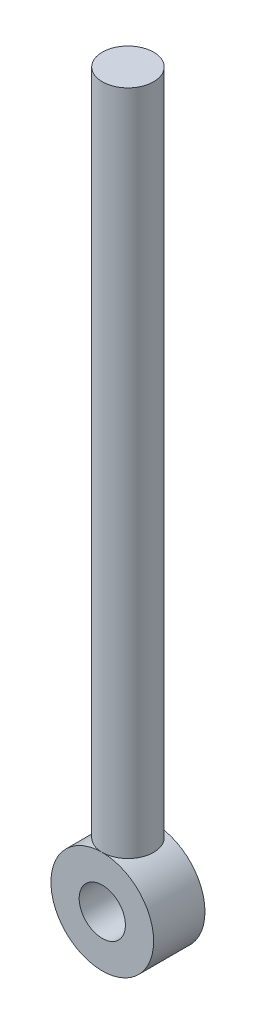
from build123d import *

# Parameters (mm, degrees)
SKETCH1_R           = 10
BOSS_EXTRUDE1_DEPTH = 5
SKETCH2_R           = 4.5
CUT_EXTRUDE1_DEPTH  = 10
SKETCH4_W           = 5
SKETCH4_H           = 130


with BuildPart() as part:
    # Sketch1 → Boss-Extrude1 (new, symmetric)
    with BuildSketch(Plane.XY):
        Circle(SKETCH1_R)
    extrude(amount=BOSS_EXTRUDE1_DEPTH, both=True)

    # Sketch2 → Cut-Extrude1 (cut)
    with BuildSketch(Plane.XY.offset(5)):
        Circle(SKETCH2_R)
    extrude(amount=-CUT_EXTRUDE1_DEPTH, mode=Mode.SUBTRACT)


with BuildPart() as body_2:
    # Sketch4 → Revolve1 (revolve)
    with BuildSketch(Plane.XY, mode=Mode.PRIVATE) as revolve1_sk:
        with Locations((2.5, 75)):
            Rectangle(SKETCH4_W, SKETCH4_H)
    revolve(revolve1_sk.sketch.rotate(Axis((0, 10, 0), (0, 1, 0)), 90), axis=Axis((0, 10, 0), (0, 1, 0)))


solid = Compound([part.part, body_2.part])
